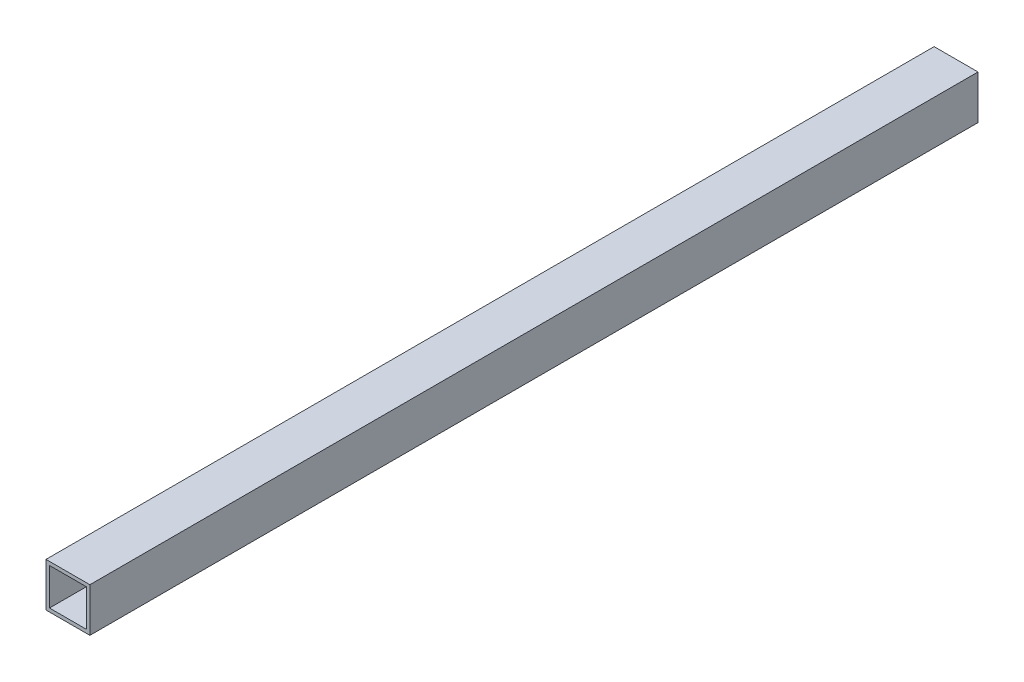
from build123d import *

# Parameters (mm, degrees)
SKETCH_1_W      = 50
SKETCH_1_H      = 50
SKETCH_1_W_2    = 42
SKETCH_1_H_2    = 42
EXTRUDE_1_DEPTH = 506


with BuildPart() as part:
    # 草图1 → 凸台-拉伸1 (new, symmetric)
    with BuildSketch(Plane.XY):
        Rectangle(SKETCH_1_W, SKETCH_1_H)
        Rectangle(SKETCH_1_W_2, SKETCH_1_H_2, mode=Mode.SUBTRACT)
    extrude(amount=EXTRUDE_1_DEPTH, both=True)


solid = part.part
